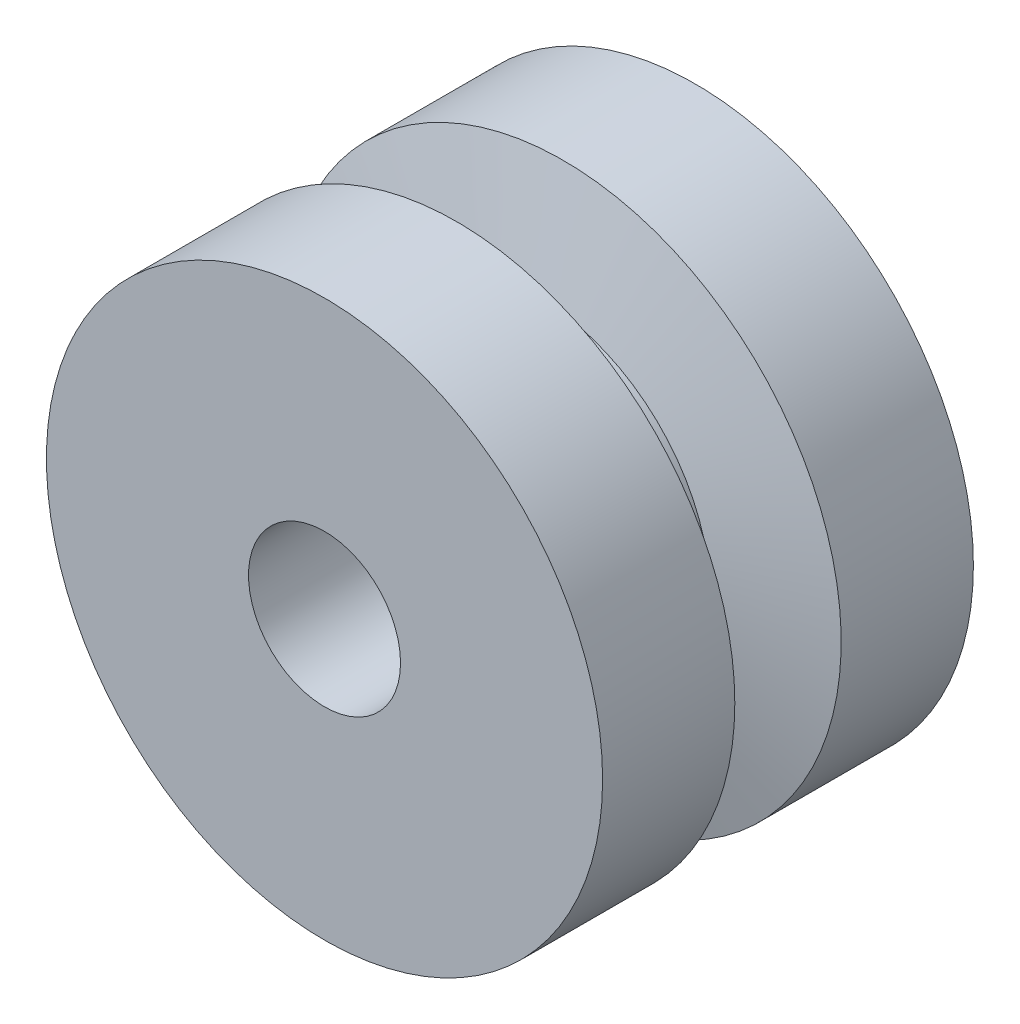
SolidWorks part; units mm, degrees
material "普通碳钢"
ref_plane "前视基准面" through (0, 0, 0) normal (0, 0, 1) x (1, 0, 0)
ref_plane "上视基准面" through (0, 0, 0) normal (0, 1, 0) x (1, 0, 0)
ref_plane "右视基准面" through (0, 0, 0) normal (1, 0, 0) x (0, 0, -1)
sketch "草图1" plane through (0, 0, 0) normal (0, 0, 1) x (1, 0, 0)
  circle A0 centre (0, 0) radius 37.5
  circle A1 centre (0, 0) radius 10.25
  dimension "D1" = 75
  dimension "D2" = 20.5
extrude "凸台-拉伸1" add sketch "草图1" along normal blind 50
sketch "草图2" plane through (0, 0, 0) normal (0, 1, 0) x (1, 0, 0)
  line L0 (37.5, -25) -> (-44.7851, -25) construction
  line L1 (37.5, -50) -> (37.5, 0) construction
  line L2 (0, 0) -> (0, -52.3687) construction
  line L3 (-38.25, -17.6488) -> (-23.25, -21.25)
  line L4 (-23.25, -21.25) -> (-23.25, -28.75)
  line L5 (-38.25, -17.6488) -> (-38.25, -32.3512)
  line L6 (-38.25, -32.3512) -> (-23.25, -28.75)
  point P11 (-23.25, -25)
  point P13 (-38.25, -25)
  dimension "D1" = 23.25
  dimension "D2" = 3.75
  dimension "D3" = 13.5
  dimension "D4" = 15
revolve "切除-旋转1" cut sketch "草图2" angle 360 about L2
ref_plane "基准面1" through (0, 32.5, 0) normal (0, 1, 0) x (1, 0, 0)
hole_wizard "M5 螺纹孔2" positions "草图4" profile "草图3" tap size "M5" standard "Iso"
sketch "草图4" plane through (0, 32.5, 0) normal (0, 1, 0) x (1, 0, 0)
  line L0 (0, 0) -> (0, -9)
  point P2 (0, -9)
  dimension "D1" = 9
sketch "草图3" plane through (0, 32.5, 9) normal (1, 0, 0) x (0, 0, 1)
  line L0 (0, 0) -> (0, 31.2618)
  line L1 (0, 31.2618) -> (2.1, 30)
  line L2 (2.1, 30) -> (2.1, 0)
  line L5 (2.1, 0) -> (0, 0)
  line L10 (0, 31.2618) -> (-2.1, 30) construction
  line L11 (0, -6.35) -> (0, 107.95) construction
  dimension "螺纹孔钻头直径" = 4.2
  dimension "螺纹孔钻头深度" = 30
  dimension "导头角度" = 118
cosmetic thread "孔螺蚊线1" parameters "D1"=22.7, "D2"=6
ref_plane "基准面2" through (32.5, 0, 0) normal (1, 0, 0) x (0, 0, -1)
hole_wizard "M5 螺纹孔1" positions "草图6" profile "草图5" tap size "M5" standard "Iso"
sketch "草图6" plane through (32.5, 0, 0) normal (1, 0, 0) x (0, 0, -1)
  line L0 (0, 0) -> (-9, 0)
  point P2 (-9, 0)
  dimension "D1" = 9
sketch "草图5" plane through (32.5, 0, 9) normal (0, 1, 0) x (0, 0, -1)
  line L0 (0, 0) -> (0, 31.2618)
  line L1 (0, 31.2618) -> (2.1, 30)
  line L2 (2.1, 30) -> (2.1, 0)
  line L5 (2.1, 0) -> (0, 0)
  line L10 (0, 31.2618) -> (-2.1, 30) construction
  line L11 (0, -6.35) -> (0, 107.95) construction
  dimension "螺纹孔钻头直径" = 4.2
  dimension "螺纹孔钻头深度" = 30
  dimension "导头角度" = 118
cosmetic thread "孔螺蚊线2" parameters "D1"=25, "D2"=5
sketch "草图7" plane through (0, 0, 0) normal (0, 0, -1) x (-1, 0, 0)
  line L0 (0, 0) -> (0, 38.7676) construction
  line L1 (-2.5, 7.95) -> (2.5, 7.95)
  line L2 (-2.5, 7.95) -> (-2.5, 12.55)
  line L3 (-2.5, 12.55) -> (2.5, 12.55)
  line L4 (2.5, 7.95) -> (2.5, 12.55)
  line L5 (-2.5, 7.95) -> (2.5, 12.55) construction
  line L6 (-2.5, 12.55) -> (2.5, 7.95) construction
  circle A0 centre (0, 0) radius 10.25 construction
  point P0 (0, 10.25)
  dimension "D1" = 5
  dimension "D2" = 4.6
